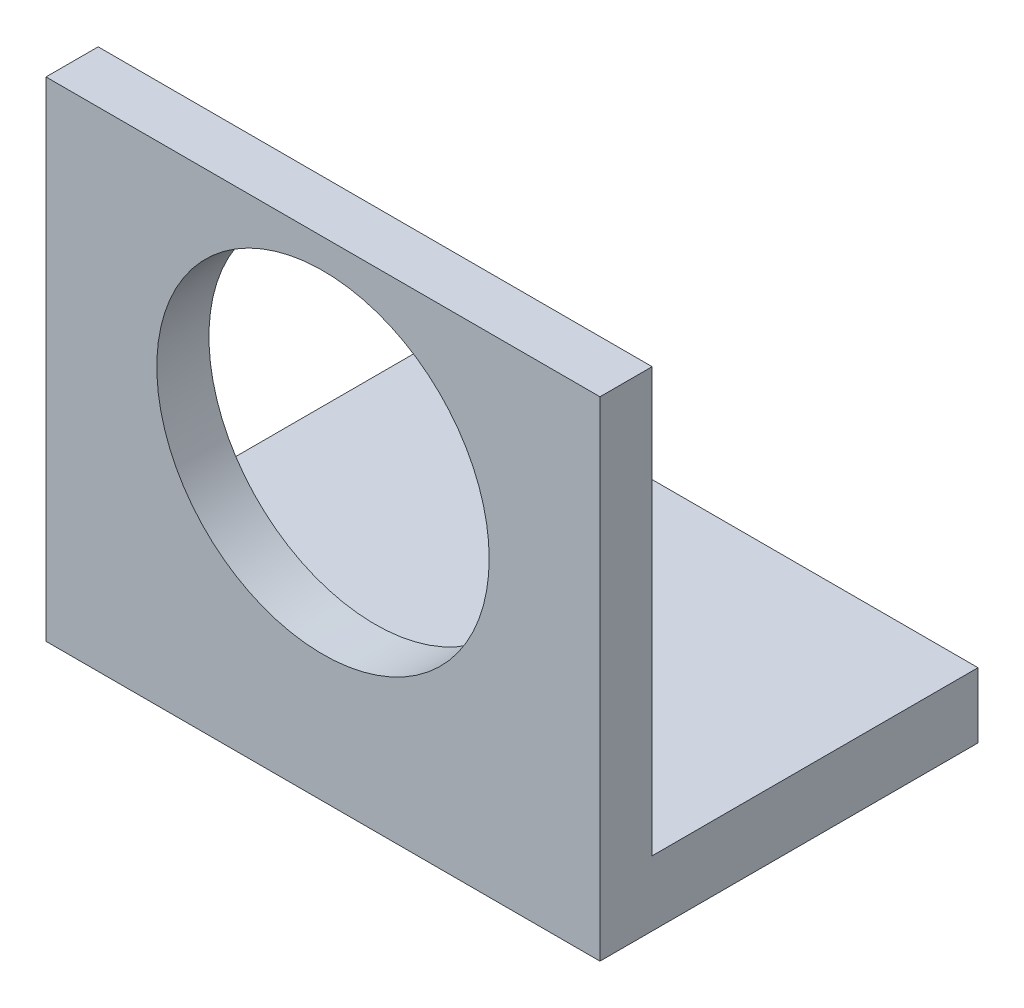
SolidWorks part; units mm, degrees
ref_plane "前视基准面" through (0, 0, 0) normal (0, 0, 1) x (1, 0, 0)
ref_plane "上视基准面" through (0, 0, 0) normal (0, 1, 0) x (1, 0, 0)
ref_plane "右视基准面" through (0, 0, 0) normal (1, 0, 0) x (0, 0, -1)
sketch "草图1" plane through (0, 0, 0) normal (0, 0, 1) x (1, 0, 0)
  line L1 (-42.5, -45) -> (42.5, -45)
  line L2 (-42.5, -45) -> (-42.5, 30)
  line L3 (-42.5, 30) -> (42.5, 30)
  line L4 (42.5, -45) -> (42.5, 30)
  line L5 (-42.5, -45) -> (42.5, 30) construction
  line L6 (-42.5, 30) -> (42.5, -45) construction
  circle A0 centre (0, 0) radius 25.5
  point P3 (0, -7.5)
  dimension "D1" = 51
  dimension "D2" = 85
  dimension "D3" = 30
  dimension "D4" = 45
extrude "凸台-拉伸1" add sketch "草图1" along normal blind 8
sketch "草图2" plane through (0, 0, 0) normal (0, 0, -1) x (-1, 0, 0)
  line L0 (42.5, 30) -> (42.5, -45) construction
  line L1 (-42.5, -45) -> (42.5, -45)
  line L2 (-42.5, -45) -> (-42.5, -35)
  line L3 (-42.5, -35) -> (42.5, -35)
  line L4 (42.5, -45) -> (42.5, -35)
  dimension "D1" = 10
extrude "凸台-拉伸2" add sketch "草图2" along normal blind 50
